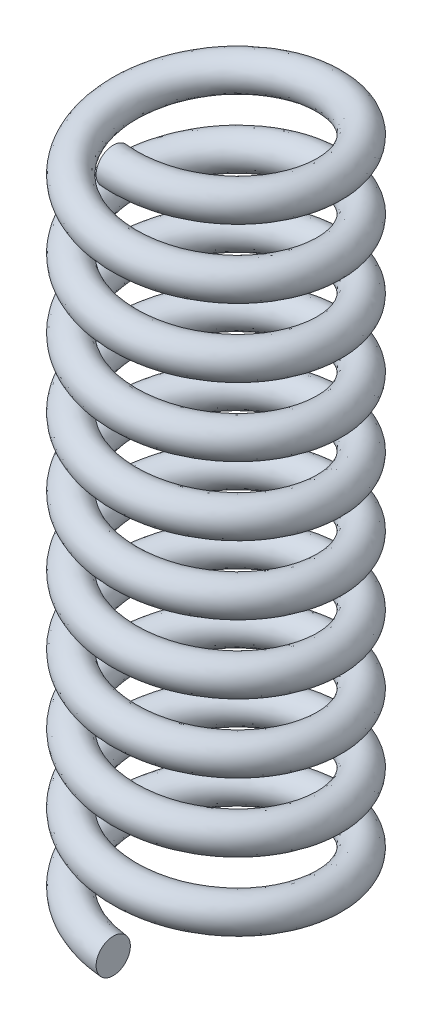
from build123d import *

# Parameters (mm, degrees)
SWEEP1_PITCH  = 2
SWEEP1_HEIGHT = 20
SWEEP1_RADIUS = 3
SKETCH1_R     = 0.5


with BuildPart() as part:
    # Sweep1: sweep along a helix
    with BuildLine() as sweep1_path:
        Helix(SWEEP1_PITCH, SWEEP1_HEIGHT, SWEEP1_RADIUS, center=(0, 0, 0), direction=(0, 1, 0), lefthand=True)
    # Sketch1 → Sweep1 (sweep)
    with BuildSketch(Plane.XY):
        with Locations((3, 0)):
            Circle(SKETCH1_R)
    sweep(path=sweep1_path.line, is_frenet=True)


solid = part.part
